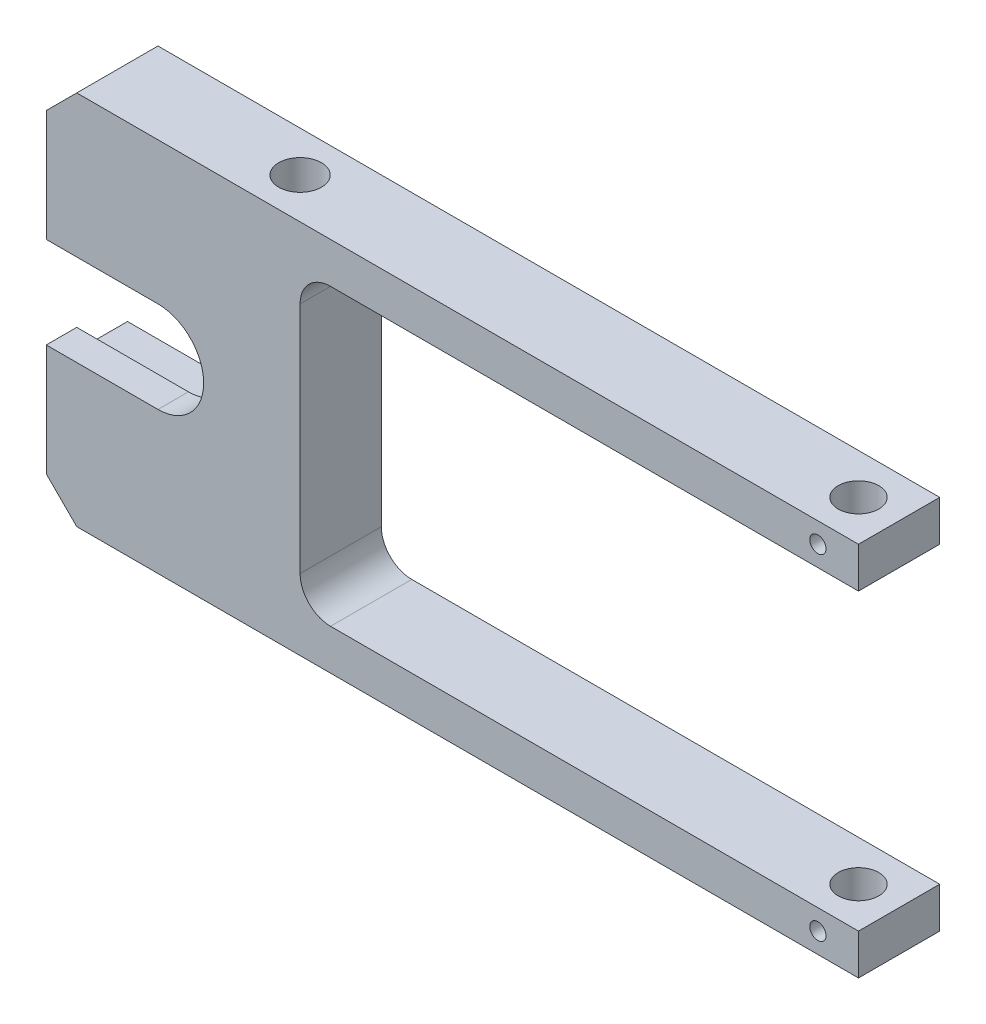
SolidWorks part; units mm, degrees
ref_plane "前视基准面" through (0, 0, 0) normal (0, 0, 1) x (1, 0, 0)
ref_plane "上视基准面" through (0, 0, 0) normal (0, 1, 0) x (1, 0, 0)
ref_plane "右视基准面" through (0, 0, 0) normal (1, 0, 0) x (0, 0, -1)
sketch "草图1" plane through (0, 0, 0) normal (0, 0, 1) x (1, 0, 0)
  line L0 (0, 0) -> (0, 14.5)
  line L1 (0, 14.5) -> (55, 14.5)
  line L2 (55, 14.5) -> (55, 18.5)
  line L3 (55, 18.5) -> (-25, 18.5)
  line L4 (-25, 18.5) -> (-25, -18.5)
  line L5 (-25, -18.5) -> (55, -18.5)
  line L6 (55, -18.5) -> (55, -14.5)
  line L7 (55, -14.5) -> (0, -14.5)
  line L8 (0, -14.5) -> (0, 0)
  dimension "D1" = 29
  dimension "D2" = 4
  dimension "D3" = 55
  dimension "D4" = 25
extrude "凸台-拉伸1" add sketch "草图1" along normal mid plane 8
sketch "草图2" plane through (0, 18.5, 0) normal (0, 1, 0) x (1, 0, 0)
  line L1 (55, -4) -> (55, 4) construction
  circle A0 centre (51, 0) radius 2
  dimension "D1" = 4
  dimension "D2" = 4
extrude "切除-拉伸1" cut sketch "草图2" against normal up to surface (37 mm away) up to face at (15, -18.5, 0)
sketch "草图3" plane through (0, -18.5, 0) normal (0, -1, 0) x (1, 0, 0)
  circle A0 centre (-4, 0) radius 2.1
  dimension "D1" = 4.2
  dimension "D2" = 4
extrude "切除-拉伸2" cut sketch "草图3" against normal up to next
hole_wizard "M2 螺纹孔1" positions "3D草图1" profile "草图4" tap size "M2" standard "GB"
sketch3d "3D草图1"
  line L0 (55, -18.5, 4) -> (55, -14.5, 4) construction
  line L1 (55, -14.5, 4) -> (0, -14.5, 4) construction
  point P0 (51, -16.5, 4)
  dimension "D1" = 4
  dimension "D2" = 2
sketch "草图4" plane through (51, -16.5, 4) normal (1, 0, 0) x (0, -1, 0)
  line L0 (0, 0) -> (0, 8)
  line L1 (0, 8) -> (0.8, 8)
  line L2 (0.8, 8) -> (0.8, 0)
  line L5 (0.8, 0) -> (0, 0)
  line L11 (0, -6.35) -> (0, 107.95) construction
  dimension "通孔螺纹孔钻头直径" = 1.6
  dimension "通孔螺纹孔钻头深度" = 8
cosmetic thread "孔螺蚊线1" parameters "D2"=2
mirror "镜向1" about plane through (0, 0, 0) normal (0, 1, 0) of "M2 螺纹孔1"
sketch "草图5" plane through (0, 0, 4) normal (0, 0, 1) x (1, 0, 0)
  line L0 (-25, 4.5) -> (-14, 4.5)
  line L1 (-25, 18.5) -> (-25, -18.5) construction
  line L2 (-14, -4.5) -> (-25, -4.5)
  line L3 (-25, -4.5) -> (-25, 4.5)
  arc A0 (-14, 4.5) -> (-14, -4.5) centre (-14, 0) cw
  dimension "D1" = 4.5
  dimension "D2" = 11
extrude "切除-拉伸3" cut sketch "草图5" against normal up to next
sketch "草图6" plane through (0, 0, -4) normal (0, 0, -1) x (-1, 0, 0)
  line L4 (25, -6.5) -> (25, 6.5)
  line L6 (14, 6.5) -> (25, 6.5)
  line L7 (25, -6.5) -> (14, -6.5)
  line L8 (14, 6.5) -> (25, 6.5)
  line L9 (25, -6.5) -> (14, -6.5)
  arc A3 (14, 6.5) -> (14, -6.5) centre (14, 0) ccw
  arc A4 (14, 6.5) -> (14, -6.5) centre (14, 0) ccw
  dimension "D1" = 2
extrude "切除-拉伸4" cut sketch "草图6" against normal blind 5
fillet "圆角1" radius 3 2 edges at (0, -14.5, 0) (0, 14.5, 0)
chamfer "倒角1" distance 3 angle 45 2 edges at (-25, 18.5, 0) (-25, -18.5, 0)
